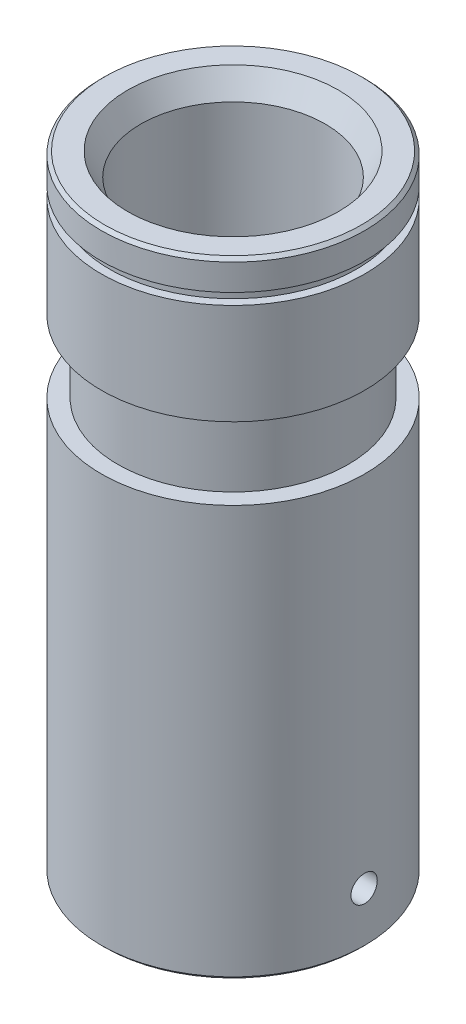
from build123d import *
from OCP.BRepFilletAPI import BRepFilletAPI_MakeChamfer

# Parameters (mm, degrees)
SKETCH_1_R            = 20
SKETCH_1_R_2          = 14
EXTRUDE_1_DEPTH       = 95
SKETCH_3_W            = 2.5
SKETCH_3_H            = 11
SKETCH_3_W_2          = 1.25
SKETCH_3_H_2          = 1.7
SKETCH_4_R            = 14
SKETCH_4_R_2          = 11
EXTRUDE_2_DEPTH       = 14
CHAMFER_1_SIZE        = 0.5
HOLE_WIZARD_4_0_4_3_D = 4
SKETCH_7_W            = 2
SKETCH_7_H            = 10
CUT_EXTRUDE_1_DEPTH   = 10
CHAMFER_2_SIZE        = 2
CHAMFER_2_SIZE2       = 3.464101615


with BuildPart() as part:
    # 草图1 → 凸台-拉伸1 (new body)
    with BuildSketch(Plane(origin=(0, 0, 0), x_dir=(1, 0, 0), z_dir=(0, 1, 0))):
        with Locations(Location((0, 0, 0), (0, 0, 270))):
            Circle(SKETCH_1_R)
        with Locations(Location((0, 0, 0), (0, 0, 270))):
            Circle(SKETCH_1_R_2, mode=Mode.SUBTRACT)
    extrude(amount=EXTRUDE_1_DEPTH)

    # 草图3 → 切除-旋转1 (revolve, cut)
    with BuildSketch(Plane.XY, mode=Mode.PRIVATE) as cut_revolve_1_sk:
        with Locations((18.75, 68)):
            Rectangle(SKETCH_3_W, SKETCH_3_H)
        with Locations((19.375, 89.65)):
            Rectangle(SKETCH_3_W_2, SKETCH_3_H_2)
    revolve(cut_revolve_1_sk.sketch.rotate(Axis((0, 0, 0), (0, 1, 0)), 90), axis=Axis((0, 0, 0), (0, 1, 0)), mode=Mode.SUBTRACT)

    # 草图4 → 凸台-拉伸2 (add)
    with BuildSketch(Plane.XZ):
        with Locations(Location((0, 0, 0), (0, 0, 270))):
            Circle(SKETCH_4_R)
        with Locations(Location((0, 0, 0), (0, 0, 270))):
            Circle(SKETCH_4_R_2, mode=Mode.SUBTRACT)
    extrude(amount=-EXTRUDE_2_DEPTH)

    # 倒角1
    chamfer_1_edges = [part.edges().sort_by_distance(p)[0] for p in [
        (0, 0, -20),
        (0, 95, -20),
    ]]
    chamfer(chamfer_1_edges, length=CHAMFER_1_SIZE)

    # Ø4.0 (4) 直径孔3 (through all)
    with Locations(Plane(origin=(20, 8, 0), x_dir=(0, 0, 1), z_dir=(1, 0, 0))):
        with Locations((0, 0)):
            Hole(HOLE_WIZARD_4_0_4_3_D / 2)

    # 草图7 → 切除-拉伸1 (cut, symmetric)
    with BuildSketch(Plane.XY):
        with Locations((-19, 35)):
            Rectangle(SKETCH_7_W, SKETCH_7_H)
    extrude(amount=CUT_EXTRUDE_1_DEPTH, both=True, mode=Mode.SUBTRACT)

    # 倒角2: one chamfer whose edges measure the first distance from different faces: ONE call of the kernel's chamfer builder (chamfer() names one face for all edges)
    chamfer_2_edges_1 = [part.edges().sort_by_distance(p)[0] for p in [
        (0, 0, 11),
    ]]
    chamfer_2_side_1 = [part.faces().sort_by_distance(p)[0] for p in [
        (0, 0, -18.948456711),
    ]]
    chamfer_2_edges_2 = [part.edges().sort_by_distance(p)[0] for p in [
        (0, 95, -14),
    ]]
    chamfer_2_side_2 = [part.faces().sort_by_distance(p)[0] for p in [
        (0, 95, -18.948456711),
    ]]
    chamfer_2 = BRepFilletAPI_MakeChamfer(part.part.solid().wrapped)
    for e in chamfer_2_edges_1:
        chamfer_2.Add(CHAMFER_2_SIZE, CHAMFER_2_SIZE2, e.wrapped, chamfer_2_side_1[0].wrapped)  # the first distance lies on this face
    for e in chamfer_2_edges_2:
        chamfer_2.Add(CHAMFER_2_SIZE, CHAMFER_2_SIZE2, e.wrapped, chamfer_2_side_2[0].wrapped)  # the first distance lies on this face
    add(Compound.cast(chamfer_2.Shape()), mode=Mode.REPLACE)


solid = part.part
